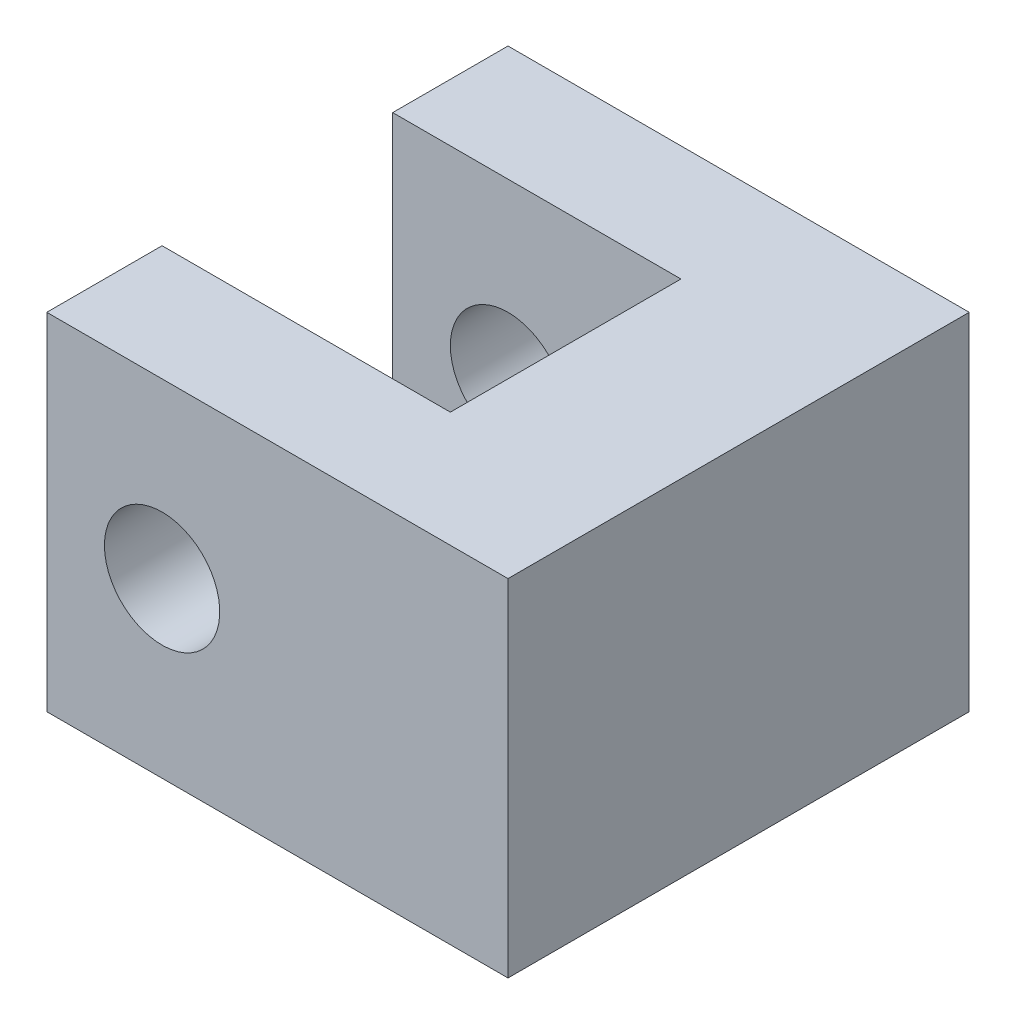
from build123d import *

# Parameters (mm, degrees)
BOSS_EXTRUDE1_DEPTH = 30
SKETCH2_R           = 5
CUT_EXTRUDE1_DEPTH  = 54.851648071


with BuildPart() as part:
    # Sketch1 → Boss-Extrude1 (new body)
    with BuildSketch(Plane(origin=(0, 0, 0), x_dir=(1, 0, 0), z_dir=(0, 1, 0))):
        Polygon((-20, 10), (-20, 20), (20, 20), (20, -20), (-20, -20), (-20, -10), (5, -10), (5, 10), align=None)
    extrude(amount=BOSS_EXTRUDE1_DEPTH)

    # Sketch2 → Cut-Extrude1 (cut, through all)
    with BuildSketch(Plane(origin=(0, 0, -20), x_dir=(-1, 0, 0), z_dir=(0, 0, -1))):
        with Locations((10, 15)):
            Circle(SKETCH2_R)
    extrude(amount=-CUT_EXTRUDE1_DEPTH, mode=Mode.SUBTRACT)


solid = part.part
